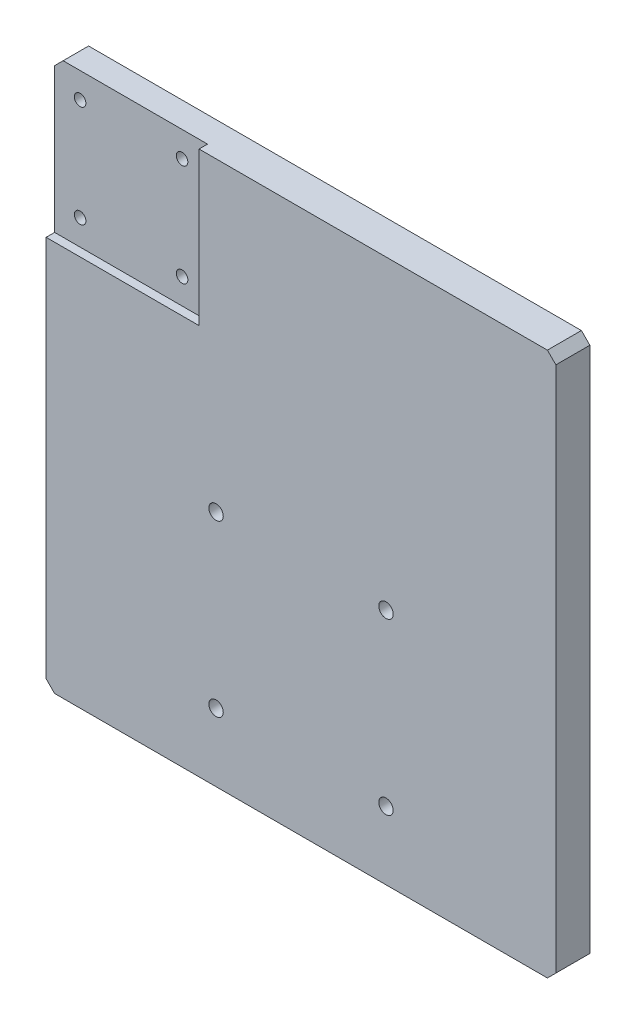
SolidWorks part; units mm, degrees
material "CuCrZr"
ref_plane "前视基准面" through (0, 0, 0) normal (0, 0, 1) x (1, 0, 0)
ref_plane "上视基准面" through (0, 0, 0) normal (0, 1, 0) x (1, 0, 0)
ref_plane "右视基准面" through (0, 0, 0) normal (1, 0, 0) x (0, 0, -1)
sketch "草图1" plane through (0, 0, 0) normal (0, 0, 1) x (1, 0, 0)
  line L5 (-150, -160) -> (150, -160)
  line L6 (-150, -160) -> (-150, 160)
  line L7 (-150, 160) -> (150, 160)
  line L8 (150, -160) -> (150, 160)
  line L9 (0, 160) -> (0, -160) construction
  line L10 (-150, 0) -> (150, 0) construction
  point P0 (0, 0)
  dimension "D1" = 300
  dimension "D2" = 320
extrude "凸台-拉伸1" add sketch "草图1" along normal mid plane 20
hole_wizard "M10 螺纹孔1" positions "草图4" profile "草图6" tap size "M10" standard "GB"
sketch "草图4" plane through (0, 0, 10) normal (0, 0, 1) x (1, 0, 0)
  line L1 (-50, -120) -> (50, -120) construction
  line L2 (-50, -120) -> (-50, -20) construction
  line L3 (-50, -20) -> (50, -20) construction
  line L4 (50, -120) -> (50, -20) construction
  line L8 (-150, -160) -> (150, -160) construction
  line L9 (0, 160) -> (0, -160) construction
  line L10 (150, 160) -> (-150, 160) construction
  point P3 (50, -20)
  point P202 (-50, -120)
  point P203 (-50, -20)
  point P204 (50, -120)
  dimension "D1" = 100
  dimension "D2" = 100
  dimension "D3" = 40
sketch "草图6" plane through (50, -20, 10) normal (1, 0, 0) x (0, -1, 0)
  line L0 (0, 0) -> (0, 17.5537)
  line L1 (0, 17.5537) -> (4.25, 15)
  line L2 (4.25, 15) -> (4.25, 0)
  line L5 (4.25, 0) -> (0, 0)
  line L10 (0, 17.5537) -> (-4.25, 15) construction
  line L11 (0, -6.35) -> (0, 107.95) construction
  dimension "螺纹孔钻头直径" = 8.5
  dimension "螺纹孔钻头深度" = 15
  dimension "导头角度" = 118
cosmetic thread "孔螺蚊线1" parameters "D1"=15, "D2"=10
cosmetic thread "孔螺蚊线2" parameters "D1"=15, "D2"=10
cosmetic thread "孔螺蚊线3" parameters "D1"=15, "D2"=10
cosmetic thread "孔螺蚊线4" parameters "D1"=15, "D2"=10
sketch "草图7" plane through (0, 0, 10) normal (0, 0, 1) x (1, 0, 0)
  line L1 (-150, 160) -> (-150, -160) construction
  line L3 (0, 160) -> (0, -160) construction
  line L4 (-150, 160) -> (-60, 160)
  line L5 (-150, 160) -> (-150, 70)
  line L6 (-150, 70) -> (-60, 70)
  line L7 (-60, 160) -> (-60, 70)
  line L8 (150, 160) -> (-150, 160) construction
  line L9 (-150, -160) -> (150, -160) construction
  dimension "D1" = 90
  dimension "D2" = 90
  dimension "D3" = 0
extrude "切除-拉伸1" cut sketch "草图7" against normal blind 5
hole_wizard "M8 螺纹孔1" positions "草图8" profile "草图9" tap size "M8" standard "GB"
sketch "草图8" plane through (0, 0, 5) normal (0, 0, 1) x (1, 0, 0)
  line L0 (-60, 115) -> (-150, 115) construction
  line L1 (-60, 70) -> (-60, 160) construction
  line L2 (-150, 160) -> (-150, 70) construction
  line L4 (-135, 85) -> (-75, 85) construction
  line L5 (-135, 85) -> (-135, 145) construction
  line L6 (-135, 145) -> (-75, 145) construction
  line L7 (-75, 85) -> (-75, 145) construction
  line L8 (-105, 145) -> (-105, 85) construction
  line L9 (-135, 115) -> (-75, 115) construction
  line L10 (-150, 70) -> (-150, -160) construction
  point P9 (-75, 145)
  point P202 (-135, 85)
  point P203 (-135, 145)
  point P204 (-75, 85)
  dimension "D1" = 60
  dimension "D2" = 60
  dimension "D3" = 15
sketch "草图9" plane through (-75, 85, 5) normal (1, 0, 0) x (0, -1, 0)
  line L0 (0, 0) -> (0, 12.0429)
  line L1 (0, 12.0429) -> (3.4, 10)
  line L2 (3.4, 10) -> (3.4, 0)
  line L5 (3.4, 0) -> (0, 0)
  line L10 (0, 12.0429) -> (-3.4, 10) construction
  line L11 (0, -6.35) -> (0, 107.95) construction
  dimension "螺纹孔钻头直径" = 6.8
  dimension "螺纹孔钻头深度" = 10
  dimension "导头角度" = 118
cosmetic thread "孔螺蚊线5" parameters "D1"=10, "D2"=8
cosmetic thread "孔螺蚊线6" parameters "D1"=10, "D2"=8
cosmetic thread "孔螺蚊线7" parameters "D1"=10, "D2"=8
cosmetic thread "孔螺蚊线8" parameters "D1"=10, "D2"=8
chamfer "倒角1" distance 5 angle 45 4 edges at (-150, -160, 0) (150, -160, 0) (150, 160, 0) (-150, 160, -2.5)
